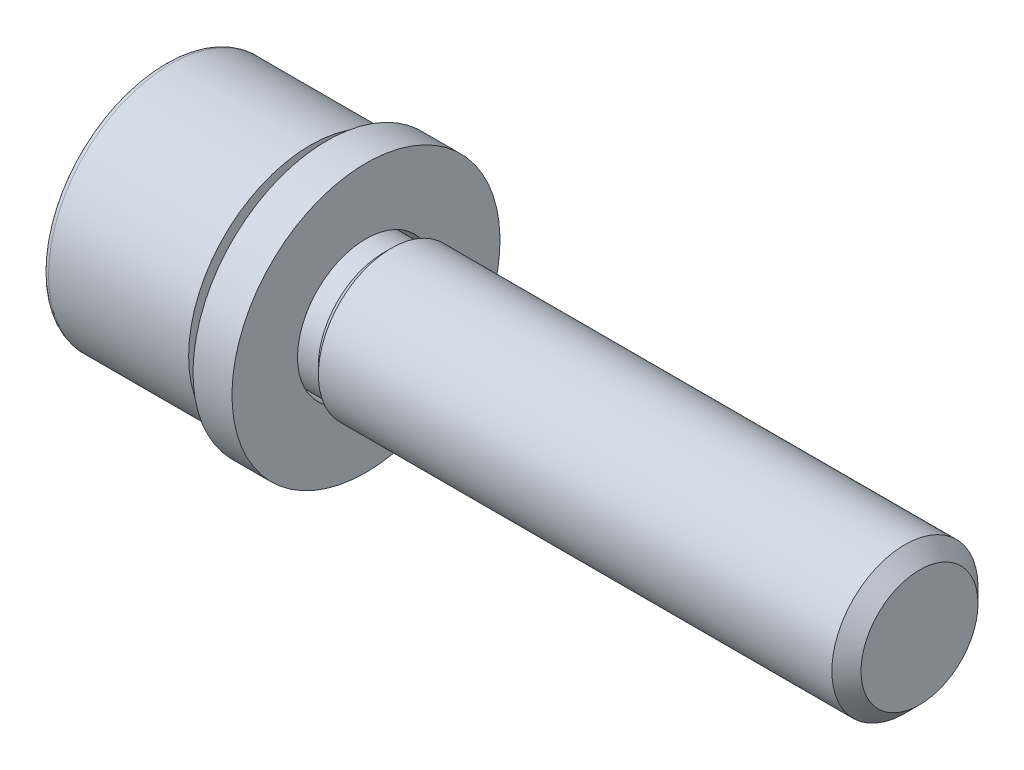
from build123d import *

# Parameters (mm, degrees)
CUT_EXTRUDE1_DEPTH = 3.7
FILLET1_R          = 0.25
SKETCH11_W         = 1.6
SKETCH11_H         = 2.69
CHAMFER1_SIZE      = 0.6


with BuildPart() as part:
    # Sketch1 → Base-Revolve (revolve)
    with BuildSketch(Plane.XY, mode=Mode.PRIVATE) as base_revolve_sk:
        with BuildLine():
            Line((0, 0), (0, 5))
            Line((0, 5), (6, 5))
            Line((6, 5), (6, 3.4))
            ThreePointArc((6, 3.4), (6.016725023, 3.310095689), (6.064662281, 3.232220591))
            Line((6.064662281, 3.232220591), (6.494662281, 2.757220591))
            ThreePointArc((6.494662281, 2.757220591), (6.57862163, 2.696477734), (6.68, 2.675))
            Line((6.68, 2.675), (9, 2.675))
            Line((9, 2.675), (9.325, 3))
            Line((9.325, 3), (31, 3))
            Line((31, 3), (31, 0))
            Line((31, 0), (0, 0))
        make_face()
    revolve(base_revolve_sk.sketch.rotate(Axis((0, 0, 0), (-1, 0, 0)), 90), axis=Axis((0, 0, 0), (-1, 0, 0)))

    # Sketch2 → Cut-Extrude1 (cut)
    with BuildSketch(Plane.ZY):
        Polygon((2.476832655, -1.43), (2.476832655, 1.43), (0, 2.86), (-2.476832655, 1.43), (-2.476832655, -1.43), (0, -2.86), align=None)
    extrude(amount=-CUT_EXTRUDE1_DEPTH, mode=Mode.SUBTRACT)

    # Sketch13 → Cut-Revolve4 (revolve, cut)
    with BuildSketch(Plane.XY):
        Polygon((0, 2.86), (0.383167345, 2.476832655), (0, 2.476832655), align=None)
    revolve(axis=Axis((0, 0, 0), (-1, 0, 0)), mode=Mode.SUBTRACT)

    # Sketch16 → Cut-Revolve5 (revolve, cut)
    with BuildSketch(Plane.XY, mode=Mode.PRIVATE) as cut_revolve5_sk:
        Polygon((5.35122177, 0), (3.7, 2.86), (3.7, 0), align=None)
    revolve(cut_revolve5_sk.sketch.rotate(Axis((3.7, 0, 0), (1, 0, 0)), 180), axis=Axis((3.7, 0, 0), (1, 0, 0)), mode=Mode.SUBTRACT)

    # Fillet1
    fillet1_edges = [part.edges().sort_by_distance(p)[0] for p in [
        (0, 0, 5),
    ]]
    fillet(fillet1_edges, radius=FILLET1_R)

    # Chamfer1
    chamfer1_edges = [part.edges().sort_by_distance(p)[0] for p in [
        (31, 0, 3),
    ]]
    chamfer(chamfer1_edges, length=CHAMFER1_SIZE)


with BuildPart() as body_2:
    # Sketch11 → Revolve1 (revolve)
    with BuildSketch(Plane.XY, mode=Mode.PRIVATE) as revolve1_sk:
        with Locations((7.48, 4.155)):
            Rectangle(SKETCH11_W, SKETCH11_H)
    revolve(revolve1_sk.sketch.rotate(Axis((0, 0, 0), (1, 0, 0)), 180), axis=Axis((0, 0, 0), (1, 0, 0)))


solid = Compound([part.part, body_2.part])
